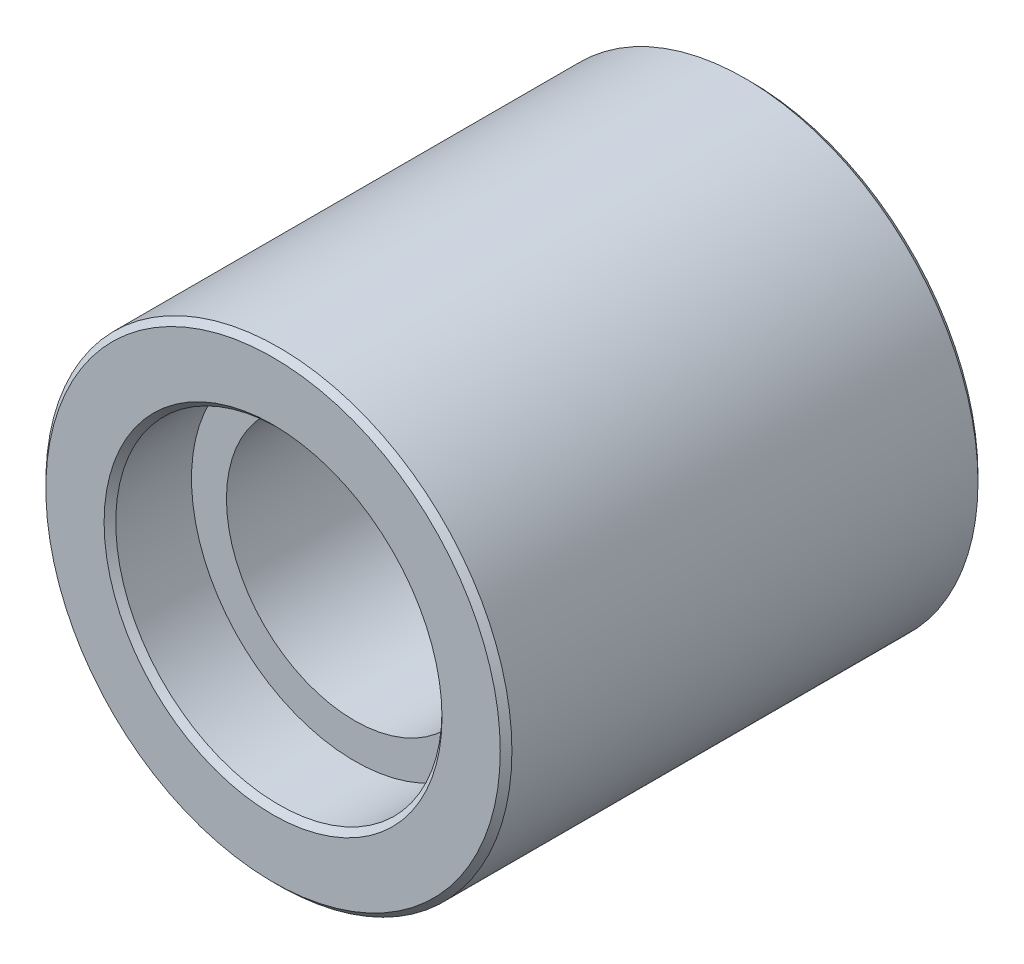
SolidWorks part; units mm, degrees
ref_plane "前视基准面" through (0, 0, 0) normal (0, 0, 1) x (1, 0, 0)
ref_plane "上视基准面" through (0, 0, 0) normal (0, 1, 0) x (1, 0, 0)
ref_plane "右视基准面" through (0, 0, 0) normal (1, 0, 0) x (0, 0, -1)
sketch "草图2" plane through (0, 0, 0) normal (0, 0, 1) x (1, 0, 0)
  circle A0 centre (0, 0) radius 20
  circle A1 centre (0, 0) radius 11
  dimension "D1" = 40
  dimension "D2" = 22
extrude "凸台-拉伸1" add sketch "草图2" along normal mid plane 41
sketch "草图3" plane through (0, 0, 20.5) normal (0, 0, 1) x (1, 0, 0)
  circle A0 centre (0, 0) radius 14
  dimension "D1" = 28
extrude "切除-拉伸1" cut sketch "草图3" against normal blind 7
mirror "镜向6" about plane through (0, 0, 0) normal (0, 0, 1) of "切除-拉伸1"
chamfer "倒角3" distance 0.5 angle 45 4 edges at (14, 0, 20.5) (14, 0, -20.5) (20, 0, 20.5) (20, 0, -20.5)
